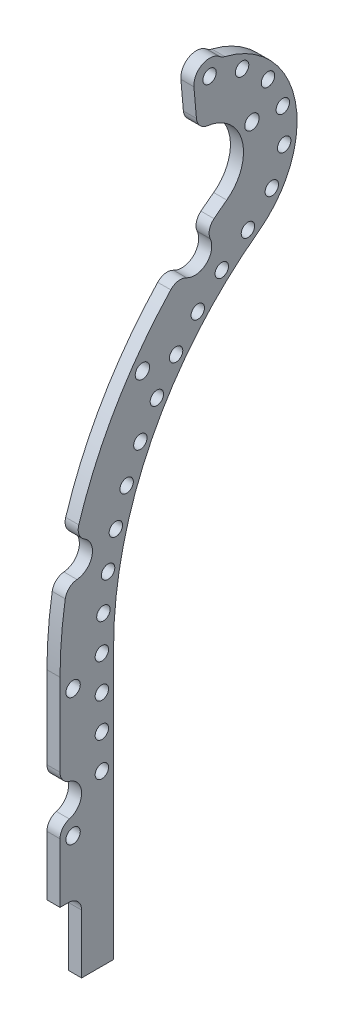
from build123d import *

# Parameters (mm, degrees)
SKETCH_3_R      = 1.025
SKETCH_3_R_2    = 1.1
EXTRUDE_1_DEPTH = 1
FILLET_R2_1_R   = 2


with BuildPart() as part:
    # 草图3 → 凸台-拉伸1 (new, symmetric)
    with BuildSketch(Plane(origin=(0, 0, 0), x_dir=(0, 0, -1), z_dir=(1, 0, 0))):
        with BuildLine():
            Line((-17.7, 0), (-17.7, -14.496003195))
            ThreePointArc((-17.7, -14.496003195), (-14.4, -17), (-17.7, -19.503996805))
            Line((-17.7, -19.503996805), (-17.7, -30.5))
            Line((-17.7, -30.5), (-14.4, -30.5))
            Line((-14.4, -30.5), (-14.4, -41.5))
            Line((-14.4, -41.5), (-9.5, -41.5))
            Line((-9.5, -41.5), (-9.5, 0))
            ThreePointArc((-9.5, 0), (-3.641643332, 24.581304561), (12.673964548, 43.877983453))
            ThreePointArc((12.673964548, 43.877983453), (18.238631052, 58.649993458), (7.015444369, 69.750348117))
            ThreePointArc((7.015444369, 69.750348117), (4.259457791, 70.419913806), (2.78947036, 67.994441237))
            Line((2.78947036, 67.994441237), (3.330713342, 61.80800564))
            ThreePointArc((3.330713342, 61.80800564), (9.932048157, 57.868608346), (7.810230773, 50.479808487))
            ThreePointArc((7.810230773, 50.479808487), (6.044157033, 49.12974963), (4.327051221, 47.71793413))
            ThreePointArc((4.327051221, 47.71793413), (4.683637937, 43.62282602), (0.629267836, 44.300430327))
            ThreePointArc((0.629267836, 44.300430327), (-9.150529626, 31.607121685), (-15.393591082, 16.849455665))
            ThreePointArc((-15.393591082, 16.849455665), (-12.809785788, 13.652423491), (-16.550868347, 11.949083889))
            ThreePointArc((-16.550868347, 11.949083889), (-17.412055908, 6.002106075), (-17.7, 0))
        make_face()
        with Locations((5.180337635, 68.203615019)):
            Circle(SKETCH_3_R, mode=Mode.SUBTRACT)
        with Locations((-15.7, -22)):
            Circle(SKETCH_3_R_2, mode=Mode.SUBTRACT)
        with Locations((-15.7, -2.5)):
            Circle(SKETCH_3_R_2, mode=Mode.SUBTRACT)
        with Locations((-5.092901527, 34.281062069)):
            Circle(SKETCH_3_R_2, mode=Mode.SUBTRACT)
        with Locations((11.666982528, 58.902824492)):
            Circle(SKETCH_3_R_2, mode=Mode.SUBTRACT)
        with Locations((10.158048255, 66.699488368)):
            Circle(SKETCH_3_R, mode=Mode.SUBTRACT)
        with Locations((14.115687733, 63.326494185)):
            Circle(SKETCH_3_R, mode=Mode.SUBTRACT)
        with Locations((16.389764399, 58.650109329)):
            Circle(SKETCH_3_R, mode=Mode.SUBTRACT)
        with Locations((16.599033086, 53.454321938)):
            Circle(SKETCH_3_R, mode=Mode.SUBTRACT)
        with Locations((14.708410246, 48.610197117)):
            Circle(SKETCH_3_R, mode=Mode.SUBTRACT)
        with Locations((11.051599939, 44.913206669)):
            Circle(SKETCH_3_R, mode=Mode.SUBTRACT)
        with Locations((7.05254031, 41.589425376)):
            Circle(SKETCH_3_R, mode=Mode.SUBTRACT)
        with Locations((3.377202973, 37.9108529)):
            Circle(SKETCH_3_R, mode=Mode.SUBTRACT)
        with Locations((0.056941504, 33.908870419)):
            Circle(SKETCH_3_R, mode=Mode.SUBTRACT)
        with Locations((-2.879919599, 29.617618054)):
            Circle(SKETCH_3_R, mode=Mode.SUBTRACT)
        with Locations((-5.408326555, 25.073703633)):
            Circle(SKETCH_3_R, mode=Mode.SUBTRACT)
        with Locations((-7.506710024, 20.315890394)):
            Circle(SKETCH_3_R, mode=Mode.SUBTRACT)
        with Locations((-9.157169108, 15.384766302)):
            Circle(SKETCH_3_R, mode=Mode.SUBTRACT)
        with Locations((-10.345624069, 10.322397804)):
            Circle(SKETCH_3_R, mode=Mode.SUBTRACT)
        with Locations((-11.06193643, 5.171970967)):
            Circle(SKETCH_3_R, mode=Mode.SUBTRACT)
        with Locations((-11.3, -0.022576726)):
            Circle(SKETCH_3_R, mode=Mode.SUBTRACT)
        with Locations((-11.3, -5.222576726)):
            Circle(SKETCH_3_R, mode=Mode.SUBTRACT)
        with Locations((-11.3, -10.422576726)):
            Circle(SKETCH_3_R, mode=Mode.SUBTRACT)
        with Locations((-11.3, -15.622576726)):
            Circle(SKETCH_3_R, mode=Mode.SUBTRACT)
    extrude(amount=EXTRUDE_1_DEPTH, both=True)

    # R2 圆角1
    fillet_r2_1_edges = [part.edges().sort_by_distance(p)[0] for p in [
        (0, -14.496003195, 17.7),
        (0, 11.949083889, 16.550868347),
        (0, 16.849455665, 15.393591082),
        (0, 44.300430327, -0.629267836),
        (0, 47.71793413, -4.327051221),
        (0, 61.80800564, -3.330713342),
        (0, 69.750348117, -7.015444369),
        (0, -30.5, 14.4),
        (0, -19.503996805, 17.7),
    ]]
    fillet(fillet_r2_1_edges, radius=FILLET_R2_1_R)


solid = part.part
